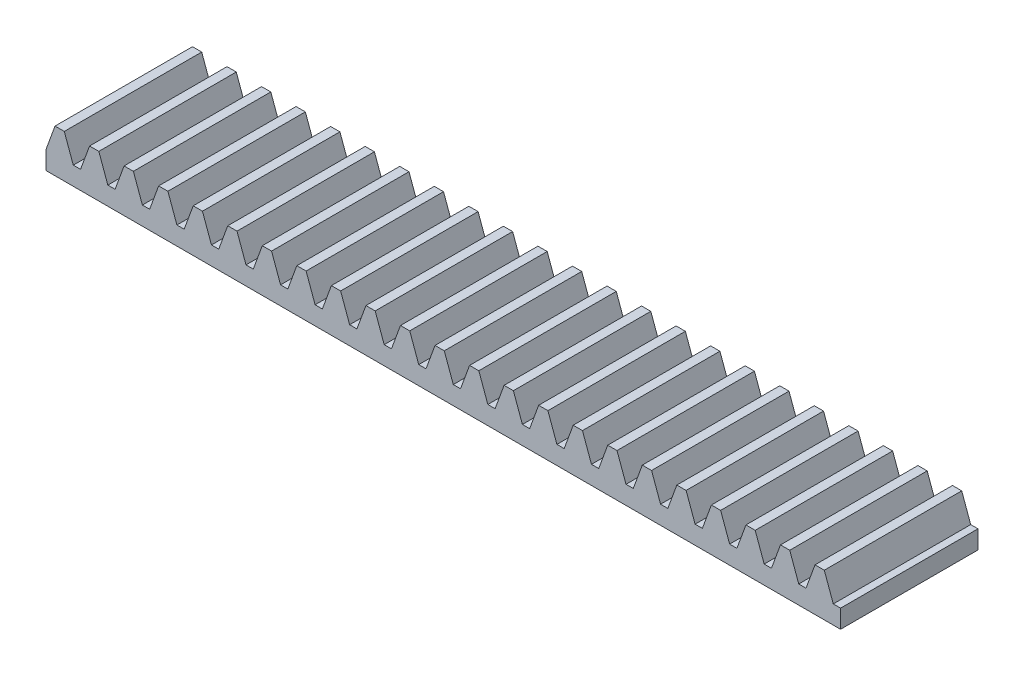
SolidWorks part; units mm, degrees
ref_plane "Front Plane" through (0, 0, 0) normal (0, 0, 1) x (1, 0, 0)
ref_plane "Top Plane" through (0, 0, 0) normal (0, 1, 0) x (1, 0, 0)
ref_plane "Right Plane" through (0, 0, 0) normal (1, 0, 0) x (0, 0, -1)
sketch "Sketch1" plane through (0, 0, 0) normal (0, 0, 1) x (1, 0, 0)
  line L0 (0, 0) -> (0, 5)
  line L1 (0, 5) -> (5, 5)
  line L2 (5, 5) -> (5, 0)
  line L3 (5, 0) -> (0, 0)
extrude "Boss-Extrude1" add sketch "Sketch1" along normal blind 150
sketch "Sketch2" plane through (0, 0, 0) normal (0, 0, 1) x (1, 0, 0)
  line L0 (0, 20) -> (9.8272, 47)
  line L1 (9.8272, 47) -> (19.9415, 47)
  line L2 (19.9415, 47) -> (29.7687, 20)
  line L3 (29.7687, 20) -> (37.6991, 20)
  line L4 (37.6991, 20) -> (47.5263, 47)
  line L5 (47.5263, 47) -> (57.6406, 47)
  line L6 (57.6406, 47) -> (67.4678, 20)
  line L7 (67.4678, 20) -> (75.3982, 20)
  line L8 (75.3982, 20) -> (85.2254, 47)
  line L9 (85.2254, 47) -> (95.3397, 47)
  line L10 (95.3397, 47) -> (105.1669, 20)
  line L11 (105.1669, 20) -> (113.0973, 20)
  line L12 (113.0973, 20) -> (122.9245, 47)
  line L13 (122.9245, 47) -> (133.0388, 47)
  line L14 (133.0388, 47) -> (142.866, 20)
  line L15 (142.866, 20) -> (150.7964, 20)
  line L16 (150.7964, 20) -> (160.6236, 47)
  line L17 (160.6236, 47) -> (170.7379, 47)
  line L18 (170.7379, 47) -> (180.5651, 20)
  line L19 (180.5651, 20) -> (188.4956, 20)
  line L20 (188.4956, 20) -> (198.3228, 47)
  line L21 (198.3228, 47) -> (208.437, 47)
  line L22 (208.437, 47) -> (218.2642, 20)
  line L23 (218.2642, 20) -> (226.1947, 20)
  line L24 (226.1947, 20) -> (236.0219, 47)
  line L25 (236.0219, 47) -> (246.1361, 47)
  line L26 (246.1361, 47) -> (255.9633, 20)
  line L27 (255.9633, 20) -> (263.8938, 20)
  line L28 (263.8938, 20) -> (273.721, 47)
  line L29 (273.721, 47) -> (283.8352, 47)
  line L30 (283.8352, 47) -> (293.6624, 20)
  line L31 (293.6624, 20) -> (301.5929, 20)
  line L32 (301.5929, 20) -> (311.4201, 47)
  line L33 (311.4201, 47) -> (321.5344, 47)
  line L34 (321.5344, 47) -> (331.3616, 20)
  line L35 (331.3616, 20) -> (339.292, 20)
  line L36 (339.292, 20) -> (349.1192, 47)
  line L37 (349.1192, 47) -> (359.2335, 47)
  line L38 (359.2335, 47) -> (369.0607, 20)
  line L39 (369.0607, 20) -> (376.9911, 20)
  line L40 (376.9911, 20) -> (386.8183, 47)
  line L41 (386.8183, 47) -> (396.9326, 47)
  line L42 (396.9326, 47) -> (406.7598, 20)
  line L43 (406.7598, 20) -> (414.6902, 20)
  line L44 (414.6902, 20) -> (424.5174, 47)
  line L45 (424.5174, 47) -> (434.6317, 47)
  line L46 (434.6317, 47) -> (444.4589, 20)
  line L47 (444.4589, 20) -> (452.3893, 20)
  line L48 (452.3893, 20) -> (462.2165, 47)
  line L49 (462.2165, 47) -> (472.3308, 47)
  line L50 (472.3308, 47) -> (482.158, 20)
  line L51 (482.158, 20) -> (490.0885, 20)
  line L52 (490.0885, 20) -> (499.9157, 47)
  line L53 (499.9157, 47) -> (510.0299, 47)
  line L54 (510.0299, 47) -> (519.8571, 20)
  line L55 (519.8571, 20) -> (527.7876, 20)
  line L56 (527.7876, 20) -> (537.6148, 47)
  line L57 (537.6148, 47) -> (547.729, 47)
  line L58 (547.729, 47) -> (557.5562, 20)
  line L59 (557.5562, 20) -> (565.4867, 20)
  line L60 (565.4867, 20) -> (575.3139, 47)
  line L61 (575.3139, 47) -> (585.4281, 47)
  line L62 (585.4281, 47) -> (595.2553, 20)
  line L63 (595.2553, 20) -> (603.1858, 20)
  line L64 (603.1858, 20) -> (613.013, 47)
  line L65 (613.013, 47) -> (623.1273, 47)
  line L66 (623.1273, 47) -> (632.9545, 20)
  line L67 (632.9545, 20) -> (640.8849, 20)
  line L68 (640.8849, 20) -> (650.7121, 47)
  line L69 (650.7121, 47) -> (660.8264, 47)
  line L70 (660.8264, 47) -> (670.6536, 20)
  line L71 (670.6536, 20) -> (678.584, 20)
  line L72 (678.584, 20) -> (688.4112, 47)
  line L73 (688.4112, 47) -> (698.5255, 47)
  line L74 (698.5255, 47) -> (708.3527, 20)
  line L75 (708.3527, 20) -> (716.2831, 20)
  line L76 (716.2831, 20) -> (726.1103, 47)
  line L77 (726.1103, 47) -> (736.2246, 47)
  line L78 (736.2246, 47) -> (746.0518, 20)
  line L79 (746.0518, 20) -> (753.9822, 20)
  line L80 (753.9822, 20) -> (763.8094, 47)
  line L81 (763.8094, 47) -> (773.9237, 47)
  line L82 (773.9237, 47) -> (783.7509, 20)
  line L83 (783.7509, 20) -> (791.6813, 20)
  line L84 (791.6813, 20) -> (801.5085, 47)
  line L85 (801.5085, 47) -> (811.6228, 47)
  line L86 (811.6228, 47) -> (821.45, 20)
  line L87 (821.45, 20) -> (829.3805, 20)
  line L88 (829.3805, 20) -> (839.2077, 47)
  line L89 (839.2077, 47) -> (849.3219, 47)
  line L90 (849.3219, 47) -> (859.1491, 20)
  line L91 (859.1491, 20) -> (867.0796, 20)
  line L92 (0, 20) -> (0, 0)
  line L93 (0, 0) -> (867.0796, 0)
  line L94 (867.0796, 0) -> (867.0796, 20)
  dimension "D1" = 23
extrude "Boss-Extrude2" add sketch "Sketch2" along normal blind 150
ref_plane "Plane1" through (490.0885, 20, 150) normal (-1, 0, 0) x (0, 0, 1)
sketch "Sketch3" plane through (0, 0, 150) normal (0, 0, 1) x (1, 0, 0)
  line L0 (-76.7689, 15.0483) -> (702.1528, 15.0483)
  circle A0 centre (496.5026, 147.5483) radius 132.5 construction
